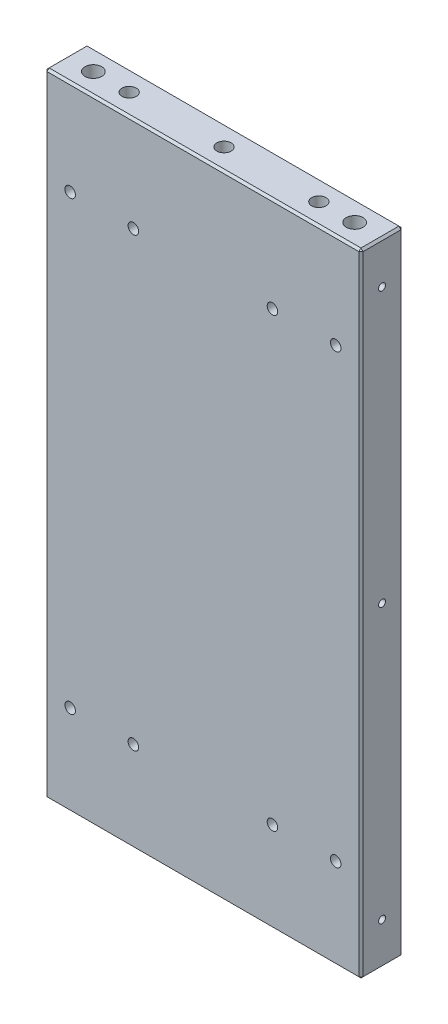
from build123d import *

# Parameters (mm, degrees)
SKETCH_1_W                  = 150
SKETCH_1_H                  = 300
EXTRUDE_1_DEPTH             = 10
CHAMFER_1_SIZE              = 1
HOLE_WIZARD_M8_1_AT_2_COUNT = 2
HOLE_WIZARD_M8_1_AT_2_PITCH = 90
HOLE_WIZARD_M8_1_AT_3_COUNT = 2
HOLE_WIZARD_M8_1_AT_3_PITCH = 45
HOLE_WIZARD_M4_1_AT_2_COUNT = 2
HOLE_WIZARD_M4_1_AT_2_PITCH = 130
HOLE_WIZARD_M4_1_AT_3_COUNT = 2
HOLE_WIZARD_M4_1_AT_3_PITCH = 260
MM_1_AT_2_COUNT             = 2
MM_1_AT_2_PITCH             = 124
HOLE_WIZARD_M6_3_D          = 5
HOLE_WIZARD_M6_4_D          = 5


with BuildPart() as part:
    # 草图1 → 凸台-拉伸1 (new, symmetric)
    with BuildSketch(Plane.XY):
        Rectangle(SKETCH_1_W, SKETCH_1_H)
    extrude(amount=EXTRUDE_1_DEPTH, both=True)

    # 倒角1
    chamfer_1_edges = [part.edges().sort_by_distance(p)[0] for p in [
        (-75, 0, 10),
        (0, -150, 10),
        (75, 0, 10),
        (0, -150, -10),
        (-75, 0, -10),
        (0, 150, -10),
        (75, 0, -10),
        (0, 150, 10),
        (75, -150, 0),
        (-75, -150, 0),
        (-75, 150, 0),
        (75, 150, 0),
    ]]
    chamfer(chamfer_1_edges, length=CHAMFER_1_SIZE)

    # 草图2 → M8 螺纹孔1 (revolve, cut)
    with BuildSketch(Plane(origin=(-45, 150, 0), x_dir=(0, 0, 1), z_dir=(1, 0, 0))):
        Polygon((0, 0), (0, 23.292926105), (3.4, 21.25), (3.4, 0), align=None)
    hole_wizard_m8_1 = revolve(axis=Axis((-45, 156.35, 0), (0, -1, 0)), mode=Mode.SUBTRACT)

    # M8 螺纹孔1 at 2: M8 螺纹孔1 ×2
    with Locations(*[(i * HOLE_WIZARD_M8_1_AT_2_PITCH, 0, 0) for i in range(1, HOLE_WIZARD_M8_1_AT_2_COUNT)]):
        add(hole_wizard_m8_1, mode=Mode.SUBTRACT)

    # M8 螺纹孔1 at 3: M8 螺纹孔1 ×2
    with Locations(*[(i * HOLE_WIZARD_M8_1_AT_3_PITCH, 0, 0) for i in range(1, HOLE_WIZARD_M8_1_AT_3_COUNT)]):
        add(hole_wizard_m8_1, mode=Mode.SUBTRACT)

    # 草图10 → M4 螺纹孔1 (revolve, cut)
    with BuildSketch(Plane(origin=(-75, -130, 0), x_dir=(0, 0, 1), z_dir=(0, 1, 0))):
        Polygon((0, 0), (0, 12.491420021), (1.65, 11.5), (1.65, 0), align=None)
    hole_wizard_m4_1 = revolve(axis=Axis((-81.35, -130, 0), (1, 0, 0)), mode=Mode.SUBTRACT)

    # M4 螺纹孔1 at 2: M4 螺纹孔1 ×2
    with Locations(*[(0, i * HOLE_WIZARD_M4_1_AT_2_PITCH, 0) for i in range(1, HOLE_WIZARD_M4_1_AT_2_COUNT)]):
        add(hole_wizard_m4_1, mode=Mode.SUBTRACT)

    # M4 螺纹孔1 at 3: M4 螺纹孔1 ×2
    with Locations(*[(0, i * HOLE_WIZARD_M4_1_AT_3_PITCH, 0) for i in range(1, HOLE_WIZARD_M4_1_AT_3_COUNT)]):
        add(hole_wizard_m4_1, mode=Mode.SUBTRACT)

    # 镜向1: M4 螺纹孔1 across plane
    add(hole_wizard_m4_1.mirror(Plane(origin=(0, 0, 0), x_dir=(0, 0, 1), z_dir=(1, 0, 0))), mode=Mode.SUBTRACT)

    # 镜向1 copy 1 sketch → 镜向1 copy 1 (revolve, cut)
    with BuildSketch(Plane(origin=(75, 0, 0), x_dir=(0, 0, 1), z_dir=(0, 1, 0))):
        Polygon((0, 0), (0, -12.491420021), (1.65, -11.5), (1.65, 0), align=None)
    revolve(axis=Axis((81.35, 0, 0), (1, 0, 0)), mode=Mode.SUBTRACT)

    # 镜向1 copy 2 sketch → 镜向1 copy 2 (revolve, cut)
    with BuildSketch(Plane(origin=(75, 130, 0), x_dir=(0, 0, 1), z_dir=(0, 1, 0))):
        Polygon((0, 0), (0, -12.491420021), (1.65, -11.5), (1.65, 0), align=None)
    revolve(axis=Axis((81.35, 130, 0), (1, 0, 0)), mode=Mode.SUBTRACT)

    # 草图16 → 大小mm 暗销孔1 (revolve, cut)
    with BuildSketch(Plane(origin=(-62, 150, 0), x_dir=(0, 0, 1), z_dir=(1, 0, 0))):
        Polygon((0, 0), (0, 17.403442476), (4, 15), (4, 0), align=None)
    mm_1 = revolve(axis=Axis((-62, 156.35, 0), (0, -1, 0)), mode=Mode.SUBTRACT)

    # 大小mm 暗销孔1 at 2: 大小mm 暗销孔1 ×2
    with Locations(*[(i * MM_1_AT_2_PITCH, 0, 0) for i in range(1, MM_1_AT_2_COUNT)]):
        add(mm_1, mode=Mode.SUBTRACT)

    # M6 螺纹孔3 (through all)
    with Locations(Plane(origin=(0, 0, -10), x_dir=(-1, 0, 0), z_dir=(0, 0, -1))):
        with Locations((-33, 105), (-63, 105), (63, 105), (33, 105)):
            Hole(HOLE_WIZARD_M6_3_D / 2)

    # M6 螺纹孔4 (through all)
    with Locations(Plane.XY.offset(10)):
        with Locations((-33, -107), (-63, -107), (33, -107), (63, -107)):
            Hole(HOLE_WIZARD_M6_4_D / 2)

    # 镜向2: M8 螺纹孔1, 大小mm 暗销孔1 across plane
    add(hole_wizard_m8_1.mirror(Plane.ZX), mode=Mode.SUBTRACT)
    add(mm_1.mirror(Plane.ZX), mode=Mode.SUBTRACT)

    # 镜向2 copy 1 sketch → 镜向2 copy 1 (revolve, cut)
    with BuildSketch(Plane(origin=(45, -150, 0), x_dir=(0, 0, 1), z_dir=(1, 0, 0))):
        Polygon((0, 0), (0, -23.292926105), (3.4, -21.25), (3.4, 0), align=None)
    revolve(axis=Axis((45, -156.35, 0), (0, -1, 0)), mode=Mode.SUBTRACT)

    # 镜向2 copy 2 sketch → 镜向2 copy 2 (revolve, cut)
    with BuildSketch(Plane(origin=(0, -150, 0), x_dir=(0, 0, 1), z_dir=(1, 0, 0))):
        Polygon((0, 0), (0, -23.292926105), (3.4, -21.25), (3.4, 0), align=None)
    revolve(axis=Axis((0, -156.35, 0), (0, -1, 0)), mode=Mode.SUBTRACT)

    # 镜向2 copy 3 sketch → 镜向2 copy 3 (revolve, cut)
    with BuildSketch(Plane(origin=(62, -150, 0), x_dir=(0, 0, 1), z_dir=(1, 0, 0))):
        Polygon((0, 0), (0, -17.403442476), (4, -15), (4, 0), align=None)
    revolve(axis=Axis((62, -156.35, 0), (0, -1, 0)), mode=Mode.SUBTRACT)


solid = part.part
